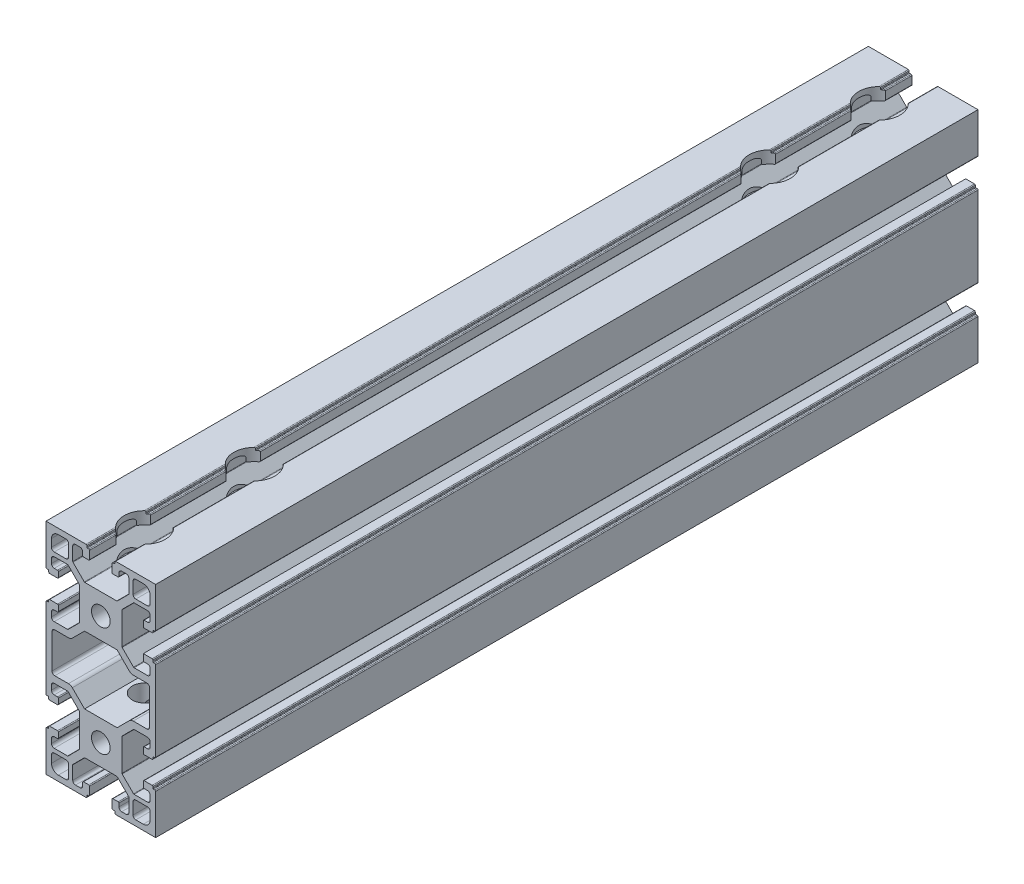
SolidWorks part; units mm, degrees
material "6061 合金"
ref_plane "前视基准面" through (0, 0, 0) normal (0, 0, 1) x (1, 0, 0)
ref_plane "上视基准面" through (0, 0, 0) normal (0, 1, 0) x (1, 0, 0)
ref_plane "右视基准面" through (0, 0, 0) normal (1, 0, 0) x (0, 0, -1)
sketch "Model" plane through (0, 0, 0) normal (0, 0, 1) x (1, 0, 0)
  line L0 (714.4099, 268.2298) -> (714.4099, 266.3298)
  line L1 (712.9099, 268.5298) -> (714.1099, 268.5298)
  line L2 (711.9099, 271.1798) -> (711.9099, 269.5298)
  line L3 (717.7679, 272.1798) -> (712.9099, 272.1798)
  line L4 (722.1221, 267.9499) -> (717.98, 272.0919)
  line L5 (722.2099, 256.1218) -> (722.2099, 267.7378)
  line L6 (717.98, 251.7677) -> (722.1221, 255.9097)
  line L7 (712.9099, 251.6798) -> (717.7679, 251.6798)
  line L8 (711.9099, 254.3298) -> (711.9099, 252.6798)
  line L9 (714.1099, 255.3298) -> (712.9099, 255.3298)
  line L10 (714.4099, 257.5298) -> (714.4099, 255.6298)
  line L11 (711.2099, 257.8298) -> (714.1099, 257.8298)
  line L12 (710.9099, 257.0298) -> (710.9099, 257.5298)
  line L13 (710.2099, 256.8298) -> (710.7099, 256.8298)
  line L14 (709.9099, 241.9298) -> (709.9099, 256.5298)
  line L15 (709.9099, 227.3298) -> (709.9099, 241.9298)
  line L16 (710.7099, 227.0298) -> (710.2099, 227.0298)
  line L17 (710.9099, 226.3298) -> (710.9099, 226.8298)
  line L18 (714.1099, 226.0298) -> (711.2099, 226.0298)
  line L19 (714.4099, 228.2298) -> (714.4099, 226.3298)
  line L20 (712.9099, 228.5298) -> (714.1099, 228.5298)
  line L21 (711.9099, 231.1798) -> (711.9099, 229.5298)
  line L22 (717.7679, 232.1798) -> (712.9099, 232.1798)
  line L23 (722.1221, 227.9499) -> (717.98, 232.0919)
  line L24 (722.2099, 216.1218) -> (722.2099, 227.7378)
  line L25 (717.98, 211.7677) -> (722.1221, 215.9097)
  line L26 (712.9099, 211.6798) -> (717.7679, 211.6798)
  line L27 (711.9099, 214.3298) -> (711.9099, 212.6798)
  line L28 (714.1099, 215.3298) -> (712.9099, 215.3298)
  line L29 (714.4099, 217.5298) -> (714.4099, 215.6298)
  line L30 (711.2099, 217.8298) -> (714.1099, 217.8298)
  line L31 (710.9099, 217.0298) -> (710.9099, 217.5298)
  line L32 (710.2099, 216.8298) -> (710.7099, 216.8298)
  line L33 (709.9099, 201.9298) -> (709.9099, 216.5298)
  line L34 (724.5099, 201.9298) -> (709.9099, 201.9298)
  line L35 (724.8099, 202.7298) -> (724.8099, 202.2298)
  line L36 (725.5099, 202.9298) -> (725.0099, 202.9298)
  line L37 (725.8099, 206.1298) -> (725.8099, 203.2298)
  line L38 (723.6099, 206.4298) -> (725.5099, 206.4298)
  line L39 (723.3099, 204.9298) -> (723.3099, 206.1298)
  line L40 (720.6599, 203.9298) -> (722.3099, 203.9298)
  line L41 (719.6599, 209.7878) -> (719.6599, 204.9298)
  line L42 (723.8898, 214.1419) -> (719.7478, 209.9999)
  line L43 (735.7179, 214.2298) -> (724.1019, 214.2298)
  line L44 (740.0721, 209.9999) -> (735.93, 214.1419)
  line L45 (740.1599, 204.9298) -> (740.1599, 209.7878)
  line L46 (737.5099, 203.9298) -> (739.1599, 203.9298)
  line L47 (736.5099, 206.1298) -> (736.5099, 204.9298)
  line L48 (734.3099, 206.4298) -> (736.2099, 206.4298)
  line L49 (734.0099, 203.2298) -> (734.0099, 206.1298)
  line L50 (734.8099, 202.9298) -> (734.3099, 202.9298)
  line L51 (735.0099, 202.2298) -> (735.0099, 202.7298)
  line L52 (749.9099, 201.9298) -> (735.3099, 201.9298)
  line L53 (749.9099, 216.5298) -> (749.9099, 201.9298)
  line L54 (749.1099, 216.8298) -> (749.6099, 216.8298)
  line L55 (748.9099, 217.5298) -> (748.9099, 217.0298)
  line L56 (745.7099, 217.8298) -> (748.6099, 217.8298)
  line L57 (745.4099, 215.6298) -> (745.4099, 217.5298)
  line L58 (746.9099, 215.3298) -> (745.7099, 215.3298)
  line L59 (747.9099, 212.6798) -> (747.9099, 214.3298)
  line L60 (742.0519, 211.6798) -> (746.9099, 211.6798)
  line L61 (737.6978, 215.9097) -> (741.8398, 211.7677)
  line L62 (737.6099, 227.7378) -> (737.6099, 216.1218)
  line L63 (741.8398, 232.0919) -> (737.6978, 227.9499)
  line L64 (746.9099, 232.1798) -> (742.0519, 232.1798)
  line L65 (747.9099, 229.5298) -> (747.9099, 231.1798)
  line L66 (745.7099, 228.5298) -> (746.9099, 228.5298)
  line L67 (745.4099, 226.3298) -> (745.4099, 228.2298)
  line L68 (748.6099, 226.0298) -> (745.7099, 226.0298)
  line L69 (748.9099, 226.8298) -> (748.9099, 226.3298)
  line L70 (749.6099, 227.0298) -> (749.1099, 227.0298)
  line L71 (749.9099, 241.9298) -> (749.9099, 227.3298)
  line L72 (749.9099, 256.5298) -> (749.9099, 241.9298)
  line L73 (749.1099, 256.8298) -> (749.6099, 256.8298)
  line L74 (748.9099, 257.5298) -> (748.9099, 257.0298)
  line L75 (745.4099, 257.8298) -> (748.6099, 257.8298)
  line L76 (745.4099, 255.3298) -> (745.4099, 257.8298)
  line L77 (746.9099, 255.3298) -> (745.4099, 255.3298)
  line L78 (747.9099, 252.6798) -> (747.9099, 254.3298)
  line L79 (742.0519, 251.6798) -> (746.9099, 251.6798)
  line L80 (737.6978, 255.9097) -> (741.8398, 251.7677)
  line L81 (737.6099, 267.7378) -> (737.6099, 256.1218)
  line L82 (741.8398, 272.0919) -> (737.6978, 267.9499)
  line L83 (746.9099, 272.1798) -> (742.0519, 272.1798)
  line L84 (747.9099, 269.5298) -> (747.9099, 271.1798)
  line L85 (745.7099, 268.5298) -> (746.9099, 268.5298)
  line L86 (745.4099, 266.3298) -> (745.4099, 268.2298)
  line L87 (748.6099, 266.0298) -> (745.7099, 266.0298)
  line L88 (748.9099, 266.8298) -> (748.9099, 266.3298)
  line L89 (749.6099, 267.0298) -> (749.1099, 267.0298)
  line L90 (749.9099, 281.9298) -> (749.9099, 267.3298)
  line L91 (735.3099, 281.9298) -> (749.9099, 281.9298)
  line L92 (735.0099, 281.1298) -> (735.0099, 281.6298)
  line L93 (734.3099, 280.9298) -> (734.8099, 280.9298)
  line L94 (734.0099, 277.7298) -> (734.0099, 280.6298)
  line L95 (736.2099, 277.4298) -> (734.3099, 277.4298)
  line L96 (736.5099, 278.9298) -> (736.5099, 277.7298)
  line L97 (739.1599, 279.9298) -> (737.5099, 279.9298)
  line L98 (740.1599, 274.0718) -> (740.1599, 278.9298)
  line L99 (735.93, 269.7177) -> (740.0721, 273.8597)
  line L100 (724.1019, 269.6298) -> (735.7179, 269.6298)
  line L101 (719.7478, 273.8597) -> (723.8898, 269.7177)
  line L102 (719.6599, 278.9298) -> (719.6599, 274.0718)
  line L103 (722.3099, 279.9298) -> (720.6599, 279.9298)
  line L104 (723.3099, 277.7298) -> (723.3099, 278.9298)
  line L105 (725.5099, 277.4298) -> (723.6099, 277.4298)
  line L106 (725.8099, 280.6298) -> (725.8099, 277.7298)
  line L107 (725.0099, 280.9298) -> (725.5099, 280.9298)
  line L108 (724.8099, 281.6298) -> (724.8099, 281.1298)
  line L109 (709.9099, 281.9298) -> (724.5099, 281.9298)
  line L110 (709.9099, 267.3298) -> (709.9099, 281.9298)
  line L111 (710.7099, 267.0298) -> (710.2099, 267.0298)
  line L112 (710.9099, 266.3298) -> (710.9099, 266.8298)
  line L113 (714.1099, 266.0298) -> (711.2099, 266.0298)
  line L114 (718.0993, 234.6798) -> (713.1099, 234.6798)
  line L115 (712.1099, 235.6798) -> (712.1099, 241.9298)
  line L116 (712.1099, 241.9298) -> (712.1099, 248.1798)
  line L117 (713.1099, 249.1798) -> (718.0993, 249.1798)
  line L118 (719.5135, 249.7656) -> (723.9777, 254.2298)
  line L119 (723.9777, 254.2298) -> (735.8422, 254.2298)
  line L120 (735.8422, 254.2298) -> (740.3064, 249.7656)
  line L121 (741.7206, 249.1798) -> (746.7099, 249.1798)
  line L122 (747.7099, 248.1798) -> (747.7099, 241.9298)
  line L123 (747.7099, 241.9298) -> (747.7099, 235.6798)
  line L124 (746.7099, 234.6798) -> (741.7206, 234.6798)
  line L125 (740.3064, 234.094) -> (735.8422, 229.6298)
  line L126 (735.8422, 229.6298) -> (723.9777, 229.6298)
  line L127 (723.9777, 229.6298) -> (719.5135, 234.094)
  line L128 (718.1599, 278.9298) -> (718.1599, 274.6798)
  line L129 (717.1599, 273.6798) -> (712.9099, 273.6798)
  line L130 (711.9099, 274.6798) -> (711.9099, 277.4298)
  line L131 (714.4099, 279.9298) -> (717.1599, 279.9298)
  line L132 (741.6599, 278.9298) -> (741.6599, 274.6798)
  line L133 (742.6599, 273.6798) -> (746.9099, 273.6798)
  line L134 (747.9099, 274.6798) -> (747.9099, 277.4298)
  line L135 (745.4099, 279.9298) -> (742.6599, 279.9298)
  line L136 (711.9099, 206.4298) -> (711.9099, 209.1798)
  line L137 (712.9099, 210.1798) -> (717.1599, 210.1798)
  line L138 (718.1599, 209.1798) -> (718.1599, 204.9298)
  line L139 (717.1599, 203.9298) -> (714.4099, 203.9298)
  line L140 (742.6599, 203.9298) -> (745.4099, 203.9298)
  line L141 (747.9099, 206.4298) -> (747.9099, 209.1798)
  line L142 (746.9099, 210.1798) -> (742.6599, 210.1798)
  line L143 (741.6599, 209.1798) -> (741.6599, 204.9298)
  arc A0 (714.1099, 266.0298) -> (714.4099, 266.3298) centre (714.1099, 266.3298) ccw
  arc A1 (714.4099, 268.2298) -> (714.1099, 268.5298) centre (714.1099, 268.2298) ccw
  arc A2 (711.9099, 269.5298) -> (712.9099, 268.5298) centre (712.9099, 269.5298) ccw
  arc A3 (712.9099, 272.1798) -> (711.9099, 271.1798) centre (712.9099, 271.1798) ccw
  arc A4 (717.98, 272.0919) -> (717.7679, 272.1798) centre (717.7679, 271.8798) ccw
  arc A5 (722.2099, 267.7378) -> (722.1221, 267.9499) centre (721.9099, 267.7378) ccw
  arc A6 (722.1221, 255.9097) -> (722.2099, 256.1218) centre (721.9099, 256.1218) ccw
  arc A7 (717.7679, 251.6798) -> (717.98, 251.7677) centre (717.7679, 251.9798) ccw
  arc A8 (711.9099, 252.6798) -> (712.9099, 251.6798) centre (712.9099, 252.6798) ccw
  arc A9 (712.9099, 255.3298) -> (711.9099, 254.3298) centre (712.9099, 254.3298) ccw
  arc A10 (714.1099, 255.3298) -> (714.4099, 255.6298) centre (714.1099, 255.6298) ccw
  arc A11 (714.4099, 257.5298) -> (714.1099, 257.8298) centre (714.1099, 257.5298) ccw
  arc A12 (711.2099, 257.8298) -> (710.9099, 257.5298) centre (711.2099, 257.5298) ccw
  arc A13 (710.7099, 256.8298) -> (710.9099, 257.0298) centre (710.7099, 257.0298) ccw
  arc A14 (710.2099, 256.8298) -> (709.9099, 256.5298) centre (710.2099, 256.5298) ccw
  arc A15 (709.9099, 227.3298) -> (710.2099, 227.0298) centre (710.2099, 227.3298) ccw
  arc A16 (710.9099, 226.8298) -> (710.7099, 227.0298) centre (710.7099, 226.8298) ccw
  arc A17 (710.9099, 226.3298) -> (711.2099, 226.0298) centre (711.2099, 226.3298) ccw
  arc A18 (714.1099, 226.0298) -> (714.4099, 226.3298) centre (714.1099, 226.3298) ccw
  arc A19 (714.4099, 228.2298) -> (714.1099, 228.5298) centre (714.1099, 228.2298) ccw
  arc A20 (711.9099, 229.5298) -> (712.9099, 228.5298) centre (712.9099, 229.5298) ccw
  arc A21 (712.9099, 232.1798) -> (711.9099, 231.1798) centre (712.9099, 231.1798) ccw
  arc A22 (717.98, 232.0919) -> (717.7679, 232.1798) centre (717.7679, 231.8798) ccw
  arc A23 (722.2099, 227.7378) -> (722.1221, 227.9499) centre (721.9099, 227.7378) ccw
  arc A24 (722.1221, 215.9097) -> (722.2099, 216.1218) centre (721.9099, 216.1218) ccw
  arc A25 (717.7679, 211.6798) -> (717.98, 211.7677) centre (717.7679, 211.9798) ccw
  arc A26 (711.9099, 212.6798) -> (712.9099, 211.6798) centre (712.9099, 212.6798) ccw
  arc A27 (712.9099, 215.3298) -> (711.9099, 214.3298) centre (712.9099, 214.3298) ccw
  arc A28 (714.1099, 215.3298) -> (714.4099, 215.6298) centre (714.1099, 215.6298) ccw
  arc A29 (714.4099, 217.5298) -> (714.1099, 217.8298) centre (714.1099, 217.5298) ccw
  arc A30 (711.2099, 217.8298) -> (710.9099, 217.5298) centre (711.2099, 217.5298) ccw
  arc A31 (710.7099, 216.8298) -> (710.9099, 217.0298) centre (710.7099, 217.0298) ccw
  arc A32 (710.2099, 216.8298) -> (709.9099, 216.5298) centre (710.2099, 216.5298) ccw
  arc A34 (724.5099, 201.9298) -> (724.8099, 202.2298) centre (724.5099, 202.2298) ccw
  arc A35 (725.0099, 202.9298) -> (724.8099, 202.7298) centre (725.0099, 202.7298) ccw
  arc A36 (725.5099, 202.9298) -> (725.8099, 203.2298) centre (725.5099, 203.2298) ccw
  arc A37 (725.8099, 206.1298) -> (725.5099, 206.4298) centre (725.5099, 206.1298) ccw
  arc A38 (723.6099, 206.4298) -> (723.3099, 206.1298) centre (723.6099, 206.1298) ccw
  arc A39 (722.3099, 203.9298) -> (723.3099, 204.9298) centre (722.3099, 204.9298) ccw
  arc A40 (719.6599, 204.9298) -> (720.6599, 203.9298) centre (720.6599, 204.9298) ccw
  arc A41 (719.7478, 209.9999) -> (719.6599, 209.7878) centre (719.9599, 209.7878) ccw
  arc A42 (724.1019, 214.2298) -> (723.8898, 214.1419) centre (724.1019, 213.9298) ccw
  arc A43 (735.93, 214.1419) -> (735.7179, 214.2298) centre (735.7179, 213.9298) ccw
  arc A44 (740.1599, 209.7878) -> (740.0721, 209.9999) centre (739.8599, 209.7878) ccw
  arc A45 (739.1599, 203.9298) -> (740.1599, 204.9298) centre (739.1599, 204.9298) ccw
  arc A46 (736.5099, 204.9298) -> (737.5099, 203.9298) centre (737.5099, 204.9298) ccw
  arc A47 (736.5099, 206.1298) -> (736.2099, 206.4298) centre (736.2099, 206.1298) ccw
  arc A48 (734.3099, 206.4298) -> (734.0099, 206.1298) centre (734.3099, 206.1298) ccw
  arc A49 (734.0099, 203.2298) -> (734.3099, 202.9298) centre (734.3099, 203.2298) ccw
  arc A50 (735.0099, 202.7298) -> (734.8099, 202.9298) centre (734.8099, 202.7298) ccw
  arc A51 (735.0099, 202.2298) -> (735.3099, 201.9298) centre (735.3099, 202.2298) ccw
  arc A53 (749.9099, 216.5298) -> (749.6099, 216.8298) centre (749.6099, 216.5298) ccw
  arc A54 (748.9099, 217.0298) -> (749.1099, 216.8298) centre (749.1099, 217.0298) ccw
  arc A55 (748.9099, 217.5298) -> (748.6099, 217.8298) centre (748.6099, 217.5298) ccw
  arc A56 (745.7099, 217.8298) -> (745.4099, 217.5298) centre (745.7099, 217.5298) ccw
  arc A57 (745.4099, 215.6298) -> (745.7099, 215.3298) centre (745.7099, 215.6298) ccw
  arc A58 (747.9099, 214.3298) -> (746.9099, 215.3298) centre (746.9099, 214.3298) ccw
  arc A59 (746.9099, 211.6798) -> (747.9099, 212.6798) centre (746.9099, 212.6798) ccw
  arc A60 (741.8398, 211.7677) -> (742.0519, 211.6798) centre (742.0519, 211.9798) ccw
  arc A61 (737.6099, 216.1218) -> (737.6978, 215.9097) centre (737.9099, 216.1218) ccw
  arc A62 (737.6978, 227.9499) -> (737.6099, 227.7378) centre (737.9099, 227.7378) ccw
  arc A63 (742.0519, 232.1798) -> (741.8398, 232.0919) centre (742.0519, 231.8798) ccw
  arc A64 (747.9099, 231.1798) -> (746.9099, 232.1798) centre (746.9099, 231.1798) ccw
  arc A65 (746.9099, 228.5298) -> (747.9099, 229.5298) centre (746.9099, 229.5298) ccw
  arc A66 (745.7099, 228.5298) -> (745.4099, 228.2298) centre (745.7099, 228.2298) ccw
  arc A67 (745.4099, 226.3298) -> (745.7099, 226.0298) centre (745.7099, 226.3298) ccw
  arc A68 (748.6099, 226.0298) -> (748.9099, 226.3298) centre (748.6099, 226.3298) ccw
  arc A69 (749.1099, 227.0298) -> (748.9099, 226.8298) centre (749.1099, 226.8298) ccw
  arc A70 (749.6099, 227.0298) -> (749.9099, 227.3298) centre (749.6099, 227.3298) ccw
  arc A71 (749.9099, 256.5298) -> (749.6099, 256.8298) centre (749.6099, 256.5298) ccw
  arc A72 (748.9099, 257.0298) -> (749.1099, 256.8298) centre (749.1099, 257.0298) ccw
  arc A73 (748.9099, 257.5298) -> (748.6099, 257.8298) centre (748.6099, 257.5298) ccw
  arc A74 (747.9099, 254.3298) -> (746.9099, 255.3298) centre (746.9099, 254.3298) ccw
  arc A75 (746.9099, 251.6798) -> (747.9099, 252.6798) centre (746.9099, 252.6798) ccw
  arc A76 (741.8398, 251.7677) -> (742.0519, 251.6798) centre (742.0519, 251.9798) ccw
  arc A77 (737.6099, 256.1218) -> (737.6978, 255.9097) centre (737.9099, 256.1218) ccw
  arc A78 (737.6978, 267.9499) -> (737.6099, 267.7378) centre (737.9099, 267.7378) ccw
  arc A79 (742.0519, 272.1798) -> (741.8398, 272.0919) centre (742.0519, 271.8798) ccw
  arc A80 (747.9099, 271.1798) -> (746.9099, 272.1798) centre (746.9099, 271.1798) ccw
  arc A81 (746.9099, 268.5298) -> (747.9099, 269.5298) centre (746.9099, 269.5298) ccw
  arc A82 (745.7099, 268.5298) -> (745.4099, 268.2298) centre (745.7099, 268.2298) ccw
  arc A83 (745.4099, 266.3298) -> (745.7099, 266.0298) centre (745.7099, 266.3298) ccw
  arc A84 (748.6099, 266.0298) -> (748.9099, 266.3298) centre (748.6099, 266.3298) ccw
  arc A85 (749.1099, 267.0298) -> (748.9099, 266.8298) centre (749.1099, 266.8298) ccw
  arc A86 (749.6099, 267.0298) -> (749.9099, 267.3298) centre (749.6099, 267.3298) ccw
  arc A88 (735.3099, 281.9298) -> (735.0099, 281.6298) centre (735.3099, 281.6298) ccw
  arc A89 (734.8099, 280.9298) -> (735.0099, 281.1298) centre (734.8099, 281.1298) ccw
  arc A90 (734.3099, 280.9298) -> (734.0099, 280.6298) centre (734.3099, 280.6298) ccw
  arc A91 (734.0099, 277.7298) -> (734.3099, 277.4298) centre (734.3099, 277.7298) ccw
  arc A92 (736.2099, 277.4298) -> (736.5099, 277.7298) centre (736.2099, 277.7298) ccw
  arc A93 (737.5099, 279.9298) -> (736.5099, 278.9298) centre (737.5099, 278.9298) ccw
  arc A94 (740.1599, 278.9298) -> (739.1599, 279.9298) centre (739.1599, 278.9298) ccw
  arc A95 (740.0721, 273.8597) -> (740.1599, 274.0718) centre (739.8599, 274.0718) ccw
  arc A96 (735.7179, 269.6298) -> (735.93, 269.7177) centre (735.7179, 269.9298) ccw
  arc A97 (723.8898, 269.7177) -> (724.1019, 269.6298) centre (724.1019, 269.9298) ccw
  arc A98 (719.6599, 274.0718) -> (719.7478, 273.8597) centre (719.9599, 274.0718) ccw
  arc A99 (720.6599, 279.9298) -> (719.6599, 278.9298) centre (720.6599, 278.9298) ccw
  arc A100 (723.3099, 278.9298) -> (722.3099, 279.9298) centre (722.3099, 278.9298) ccw
  arc A101 (723.3099, 277.7298) -> (723.6099, 277.4298) centre (723.6099, 277.7298) ccw
  arc A102 (725.5099, 277.4298) -> (725.8099, 277.7298) centre (725.5099, 277.7298) ccw
  arc A103 (725.8099, 280.6298) -> (725.5099, 280.9298) centre (725.5099, 280.6298) ccw
  arc A104 (724.8099, 281.1298) -> (725.0099, 280.9298) centre (725.0099, 281.1298) ccw
  arc A105 (724.8099, 281.6298) -> (724.5099, 281.9298) centre (724.5099, 281.6298) ccw
  arc A107 (709.9099, 267.3298) -> (710.2099, 267.0298) centre (710.2099, 267.3298) ccw
  arc A108 (710.9099, 266.8298) -> (710.7099, 267.0298) centre (710.7099, 266.8298) ccw
  arc A109 (710.9099, 266.3298) -> (711.2099, 266.0298) centre (711.2099, 266.3298) ccw
  arc A110 (712.1099, 235.6798) -> (713.1099, 234.6798) centre (713.1099, 235.6798) ccw
  arc A111 (713.1099, 249.1798) -> (712.1099, 248.1798) centre (713.1099, 248.1798) ccw
  arc A112 (718.0993, 249.1798) -> (719.5135, 249.7656) centre (718.0993, 251.1798) ccw
  arc A113 (740.3064, 249.7656) -> (741.7206, 249.1798) centre (741.7206, 251.1798) ccw
  arc A114 (747.7099, 248.1798) -> (746.7099, 249.1798) centre (746.7099, 248.1798) ccw
  arc A115 (746.7099, 234.6798) -> (747.7099, 235.6798) centre (746.7099, 235.6798) ccw
  arc A116 (741.7206, 234.6798) -> (740.3064, 234.094) centre (741.7206, 232.6798) ccw
  arc A117 (719.5135, 234.094) -> (718.0993, 234.6798) centre (718.0993, 232.6798) ccw
  circle A118 centre (729.9099, 261.9298) radius 3.4
  arc A119 (718.1599, 278.9298) -> (717.1599, 279.9298) centre (717.1599, 278.9298) ccw
  arc A120 (717.1599, 273.6798) -> (718.1599, 274.6798) centre (717.1599, 274.6798) ccw
  arc A121 (711.9099, 274.6798) -> (712.9099, 273.6798) centre (712.9099, 274.6798) ccw
  arc A122 (714.4099, 279.9298) -> (711.9099, 277.4298) centre (714.4099, 277.4298) ccw
  arc A123 (742.6599, 279.9298) -> (741.6599, 278.9298) centre (742.6599, 278.9298) ccw
  arc A124 (741.6599, 274.6798) -> (742.6599, 273.6798) centre (742.6599, 274.6798) ccw
  arc A125 (746.9099, 273.6798) -> (747.9099, 274.6798) centre (746.9099, 274.6798) ccw
  arc A126 (747.9099, 277.4298) -> (745.4099, 279.9298) centre (745.4099, 277.4298) ccw
  circle A127 centre (729.9099, 221.9298) radius 3.4
  arc A128 (712.9099, 210.1798) -> (711.9099, 209.1798) centre (712.9099, 209.1798) ccw
  arc A129 (718.1599, 209.1798) -> (717.1599, 210.1798) centre (717.1599, 209.1798) ccw
  arc A130 (717.1599, 203.9298) -> (718.1599, 204.9298) centre (717.1599, 204.9298) ccw
  arc A131 (711.9099, 206.4298) -> (714.4099, 203.9298) centre (714.4099, 206.4298) ccw
  arc A132 (741.6599, 204.9298) -> (742.6599, 203.9298) centre (742.6599, 204.9298) ccw
  arc A133 (745.4099, 203.9298) -> (747.9099, 206.4298) centre (745.4099, 206.4298) ccw
  arc A134 (747.9099, 209.1798) -> (746.9099, 210.1798) centre (746.9099, 209.1798) ccw
  arc A135 (742.6599, 210.1798) -> (741.6599, 209.1798) centre (742.6599, 209.1798) ccw
extrude "凸台-拉伸1" add sketch "Model" along normal mid plane 300
cosmetic thread "孔螺蚊线1" parameters "D1"=8, "D2"=8
cosmetic thread "孔螺蚊线2" parameters "D1"=8, "D2"=8
cosmetic thread "孔螺蚊线3" parameters "D1"=8, "D2"=8
cosmetic thread "孔螺蚊线4" parameters "D1"=8, "D2"=8
sketch "草图2" plane through (0, 281.9298, 0) normal (0, 1, 0) x (1, 0, 0)
  line L0 (724.5099, -150) -> (709.9099, -150) construction
  line L1 (709.9099, -150) -> (709.9099, 150) construction
  line L2 (749.9099, -150) -> (749.9099, 150) construction
  line L3 (749.9099, 150) -> (735.3099, 150) construction
  point P0 (729.9099, 134)
  point P1 (729.9099, 94)
  point P2 (729.9099, -134)
  point P3 (729.9099, -94)
  dimension "D1" = 16
  dimension "D2" = 20
  dimension "D3" = 20
  dimension "D4" = 40
  dimension "D5" = 20
  dimension "D6" = 20
  dimension "D7" = 16
  dimension "D8" = 40
hole_wizard "打孔尺寸(%根据)内六角圆柱头螺钉的类型2" positions "3D草图2" profile "草图3" counterbore size "M8" standard "GB" end condition through all
sketch3d "3D草图2"
  point P0 (729.9099, 281.9298, -134)
  point P3 (729.9099, 281.9298, -94)
  point P6 (729.9099, 281.9298, 94)
  point P9 (729.9099, 281.9298, 134)
sketch "草图3" plane through (729.9099, 281.9298, -134) normal (1, 0, 0) x (0, 0, 1)
  line L0 (0, 0) -> (0, 80)
  line L1 (0, 80) -> (4.5, 80)
  line L3 (4.5, 80) -> (4.5, 12.3)
  line L4 (4.5, 12.3) -> (7.5, 12.3)
  line L5 (7.5, 12.3) -> (7.5, 0)
  line L7 (7.5, 0) -> (0, 0)
  line L11 (0, -6.35) -> (0, 107.95) construction
  dimension "通孔孔直径" = 9
  dimension "通孔孔深度" = 80
  dimension "柱形沉头孔直径" = 15
  dimension "柱形沉头孔深度" = 12.3
hole_wizard "M8 螺纹孔1" positions "3D草图3" profile "草图4" tap size "M8" standard "GB"
sketch3d "3D草图3"
  line L0 (729.9099, 261.9298, 150) -> (729.9099, 261.9298, 136.9479) construction
  line L1 (729.9099, 221.9298, 150) -> (729.9099, 221.9298, 136.9479) construction
  line L2 (729.9099, 261.9298, -136.9479) -> (729.9099, 261.9298, -150) construction
  line L3 (729.9099, 221.9298, -136.9479) -> (729.9099, 221.9298, -150) construction
  point P0 (729.9099, 261.9298, 150)
  point P5 (729.9099, 221.9298, 150)
  point P9 (729.9099, 261.9298, -150)
  point P13 (729.9099, 221.9298, -150)
sketch "草图4" plane through (729.9099, 261.9298, 150) normal (1, 0, 0) x (0, -1, 0)
  line L0 (0, 0) -> (0, 12.2929)
  line L1 (0, 12.2929) -> (3.4, 10.25)
  line L2 (3.4, 10.25) -> (3.4, 0)
  line L5 (3.4, 0) -> (0, 0)
  line L10 (0, 12.2929) -> (-3.4, 10.25) construction
  line L11 (0, -6.35) -> (0, 107.95) construction
  dimension "螺纹孔钻头直径" = 6.8
  dimension "螺纹孔钻头深度" = 10.25
  dimension "导头角度" = 118
